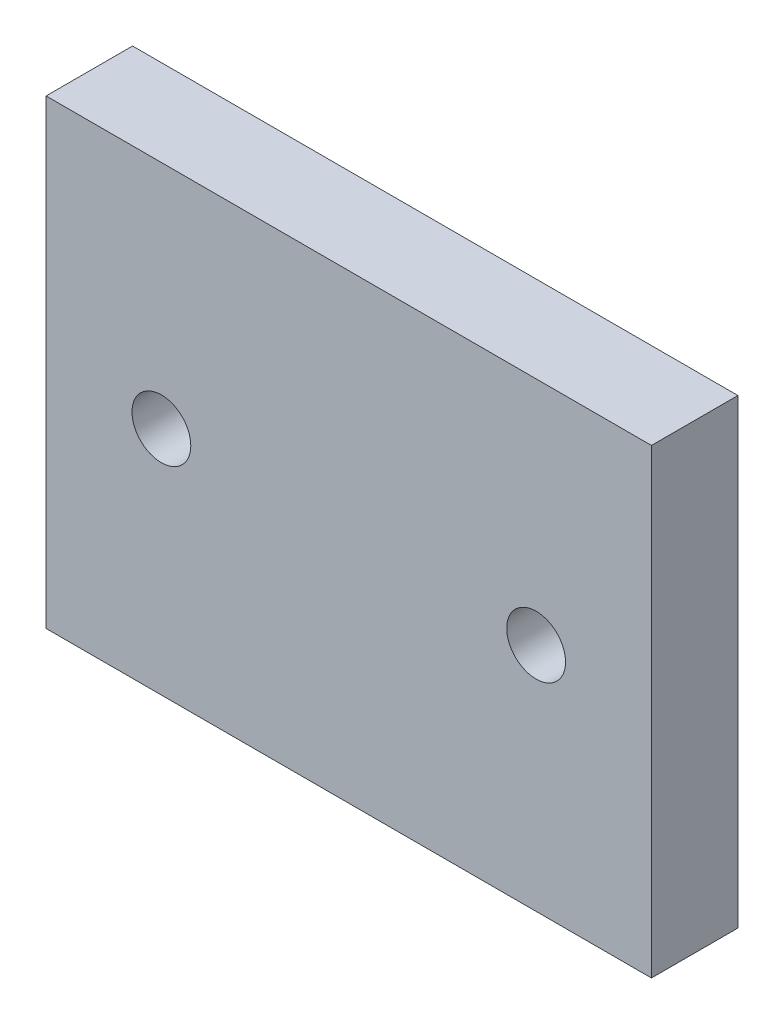
SolidWorks part; units mm, degrees
material "1023 碳钢板 (SS)"
ref_plane "前视基准面" through (0, 0, 0) normal (0, 0, 1) x (1, 0, 0)
ref_plane "上视基准面" through (0, 0, 0) normal (0, 1, 0) x (1, 0, 0)
ref_plane "右视基准面" through (0, 0, 0) normal (1, 0, 0) x (0, 0, -1)
sketch "草图1" plane through (0, 0, 0) normal (0, 0, 1) x (1, 0, 0)
  line L1 (52.5, 40) -> (-52.5, 40)
  line L2 (52.5, 40) -> (52.5, -40)
  line L3 (52.5, -40) -> (-52.5, -40)
  line L4 (-52.5, 40) -> (-52.5, -40)
  line L5 (52.5, 40) -> (-52.5, -40) construction
  line L6 (52.5, -40) -> (-52.5, 40) construction
  point P0 (0, 0)
  dimension "D1" = 105
  dimension "D2" = 80
extrude "凸台-拉伸1" add sketch "草图1" along normal blind 15
sketch "草图2" plane through (0, 0, 15) normal (0, 0, 1) x (1, 0, 0)
  circle A0 centre (-32.5, 0) radius 6.2385
  circle A1 centre (32.5, 0) radius 6.5348
  point P4 (0, 0)
  dimension "D2" = 65
  dimension "D1" = 32.5
hole_wizard "M12 螺纹孔1" positions "草图3" profile "草图4" tap size "M12" standard "ISO"
sketch "草图3" plane through (0, 0, 15) normal (0, 0, 1) x (1, 0, 0)
  point P0 (-32.5, 0)
  point P3 (32.5, 0)
sketch "草图4" plane through (-32.5, 0, 15) normal (1, 0, 0) x (0, -1, 0)
  line L0 (0, 0) -> (0, 32.3144)
  line L1 (0, 32.3144) -> (5.1, 29.25)
  line L2 (5.1, 29.25) -> (5.1, 0)
  line L5 (5.1, 0) -> (0, 0)
  line L10 (0, 32.3144) -> (-5.1, 29.25) construction
  line L11 (0, -6.35) -> (0, 107.95) construction
  dimension "螺纹孔钻头直径" = 10.2
  dimension "螺纹孔钻头深度" = 29.25
  dimension "导头角度" = 118
cosmetic thread "孔螺蚊线1" parameters "D1"=24, "D2"=12
cosmetic thread "孔螺蚊线2" parameters "D1"=24, "D2"=12
